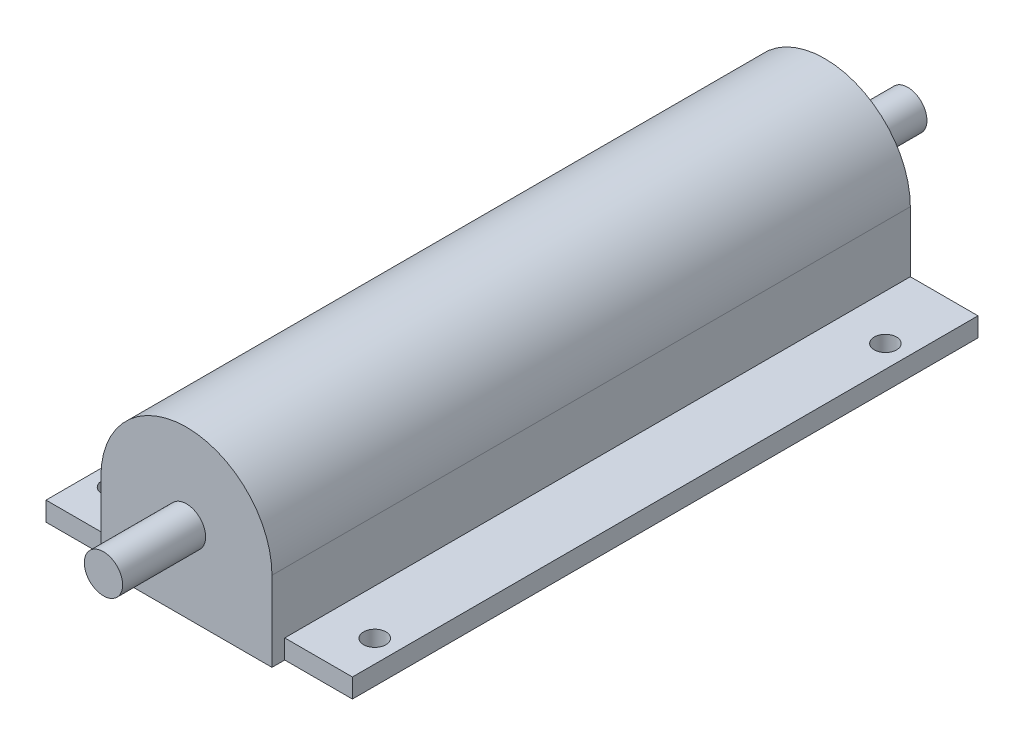
SolidWorks part; units mm, degrees
ref_plane "前视基准面" through (0, 0, 0) normal (0, 0, 1) x (1, 0, 0)
ref_plane "上视基准面" through (0, 0, 0) normal (0, 1, 0) x (1, 0, 0)
ref_plane "右视基准面" through (0, 0, 0) normal (1, 0, 0) x (0, 0, -1)
ref_plane "基准面1" through (0, 0, 49) normal (0, 0, 1) x (1, 0, 0)
sketch "草图1" plane through (0, 0, 49) normal (0, 0, 1) x (1, 0, 0)
  line L0 (-13.4, 0) -> (13.4, 0)
  line L1 (13.4, 0) -> (13.4, 12.5)
  line L2 (-13.4, 12.5) -> (-13.4, 0)
  arc A0 (13.4, 12.5) -> (-13.4, 12.5) centre (0, 12.5) ccw
extrude "凸台-拉伸1" add sketch "草图1" against normal blind 100
sketch "草图2" plane through (13.4, 0, 0) normal (1, 0, 0) x (0, 0, -1)
  line L0 (51, 0) -> (-47, 0)
  line L1 (-47, 0) -> (-47, 3)
  line L2 (-47, 3) -> (51, 3)
  line L3 (51, 3) -> (51, 0)
  line L4 (51, 0) -> (51, 12.5) construction
extrude "凸台-拉伸2" add sketch "草图2" along normal blind 10.6
sketch "草图3" plane through (0, 0, 49) normal (0, 0, 1) x (1, 0, 0)
  line L0 (-13.4, -3.4) -> (-11.4, -3.4)
  line L1 (-11.4, -3.4) -> (-11.4, 3)
  line L2 (-11.4, 3) -> (-13.4, 3)
  line L3 (-13.4, 3) -> (-13.4, -3.4)
  line L4 (24, 3) -> (13.4, 3) construction
extrude "切除-拉伸1" cut sketch "草图3" against normal through all
sketch "草图4" plane through (-11.4, 0, 0) normal (-1, 0, 0) x (0, 0, 1)
  line L0 (47, 4.9) -> (47, 0)
  line L1 (47, 0) -> (-51, 0)
  line L2 (-51, 0) -> (-51, 4.9)
  line L3 (-51, 4.9) -> (47, 4.9)
  line L4 (-51, 0) -> (-51, 3) construction
extrude "凸台-拉伸3" add sketch "草图4" along normal blind 12.6
sketch "草图5" plane through (0, 0, -51) normal (0, 0, -1) x (-1, 0, 0)
  line L0 (24, 4.9) -> (13.4, 4.9)
  line L1 (13.4, 4.9) -> (13.4, 3)
  line L2 (13.4, 3) -> (24, 3)
  line L3 (24, 3) -> (24, 4.9)
extrude "切除-拉伸2" cut sketch "草图5" against normal through all
sketch "草图6" plane through (0, 0, 49) normal (0, 0, 1) x (1, 0, 0)
  circle A0 centre (0, 12.5) radius 3
extrude "凸台-拉伸4" add sketch "草图6" along normal blind 13
sketch "草图7" plane through (0, 0, -51) normal (0, 0, -1) x (-1, 0, 0)
  circle A0 centre (0, 12.5) radius 3
extrude "凸台-拉伸5" add sketch "草图7" along normal blind 13
sketch "草图10" plane through (0, 0, 0) normal (0, -1, 0) x (1, 0, 0)
  line L1 (-20.5, 40) -> (20.5, 40) construction
  line L2 (-20.5, 40) -> (-20.5, -40) construction
  line L3 (-20.5, -40) -> (20.5, -40) construction
  line L4 (20.5, 40) -> (20.5, -40) construction
  line L5 (-20.5, 40) -> (20.5, -40) construction
  line L6 (-20.5, -40) -> (20.5, 40) construction
  circle A0 centre (-20.5, 40) radius 1.75
  circle A1 centre (20.5, 40) radius 1.75
  circle A2 centre (20.5, -40) radius 1.75
  circle A3 centre (-20.5, -40) radius 1.75
  point P0 (0, 0)
  dimension "D3" = 3.5
  dimension "D1" = 80
  dimension "D2" = 41
extrude "切除-拉伸3" cut sketch "草图10" against normal blind 10
